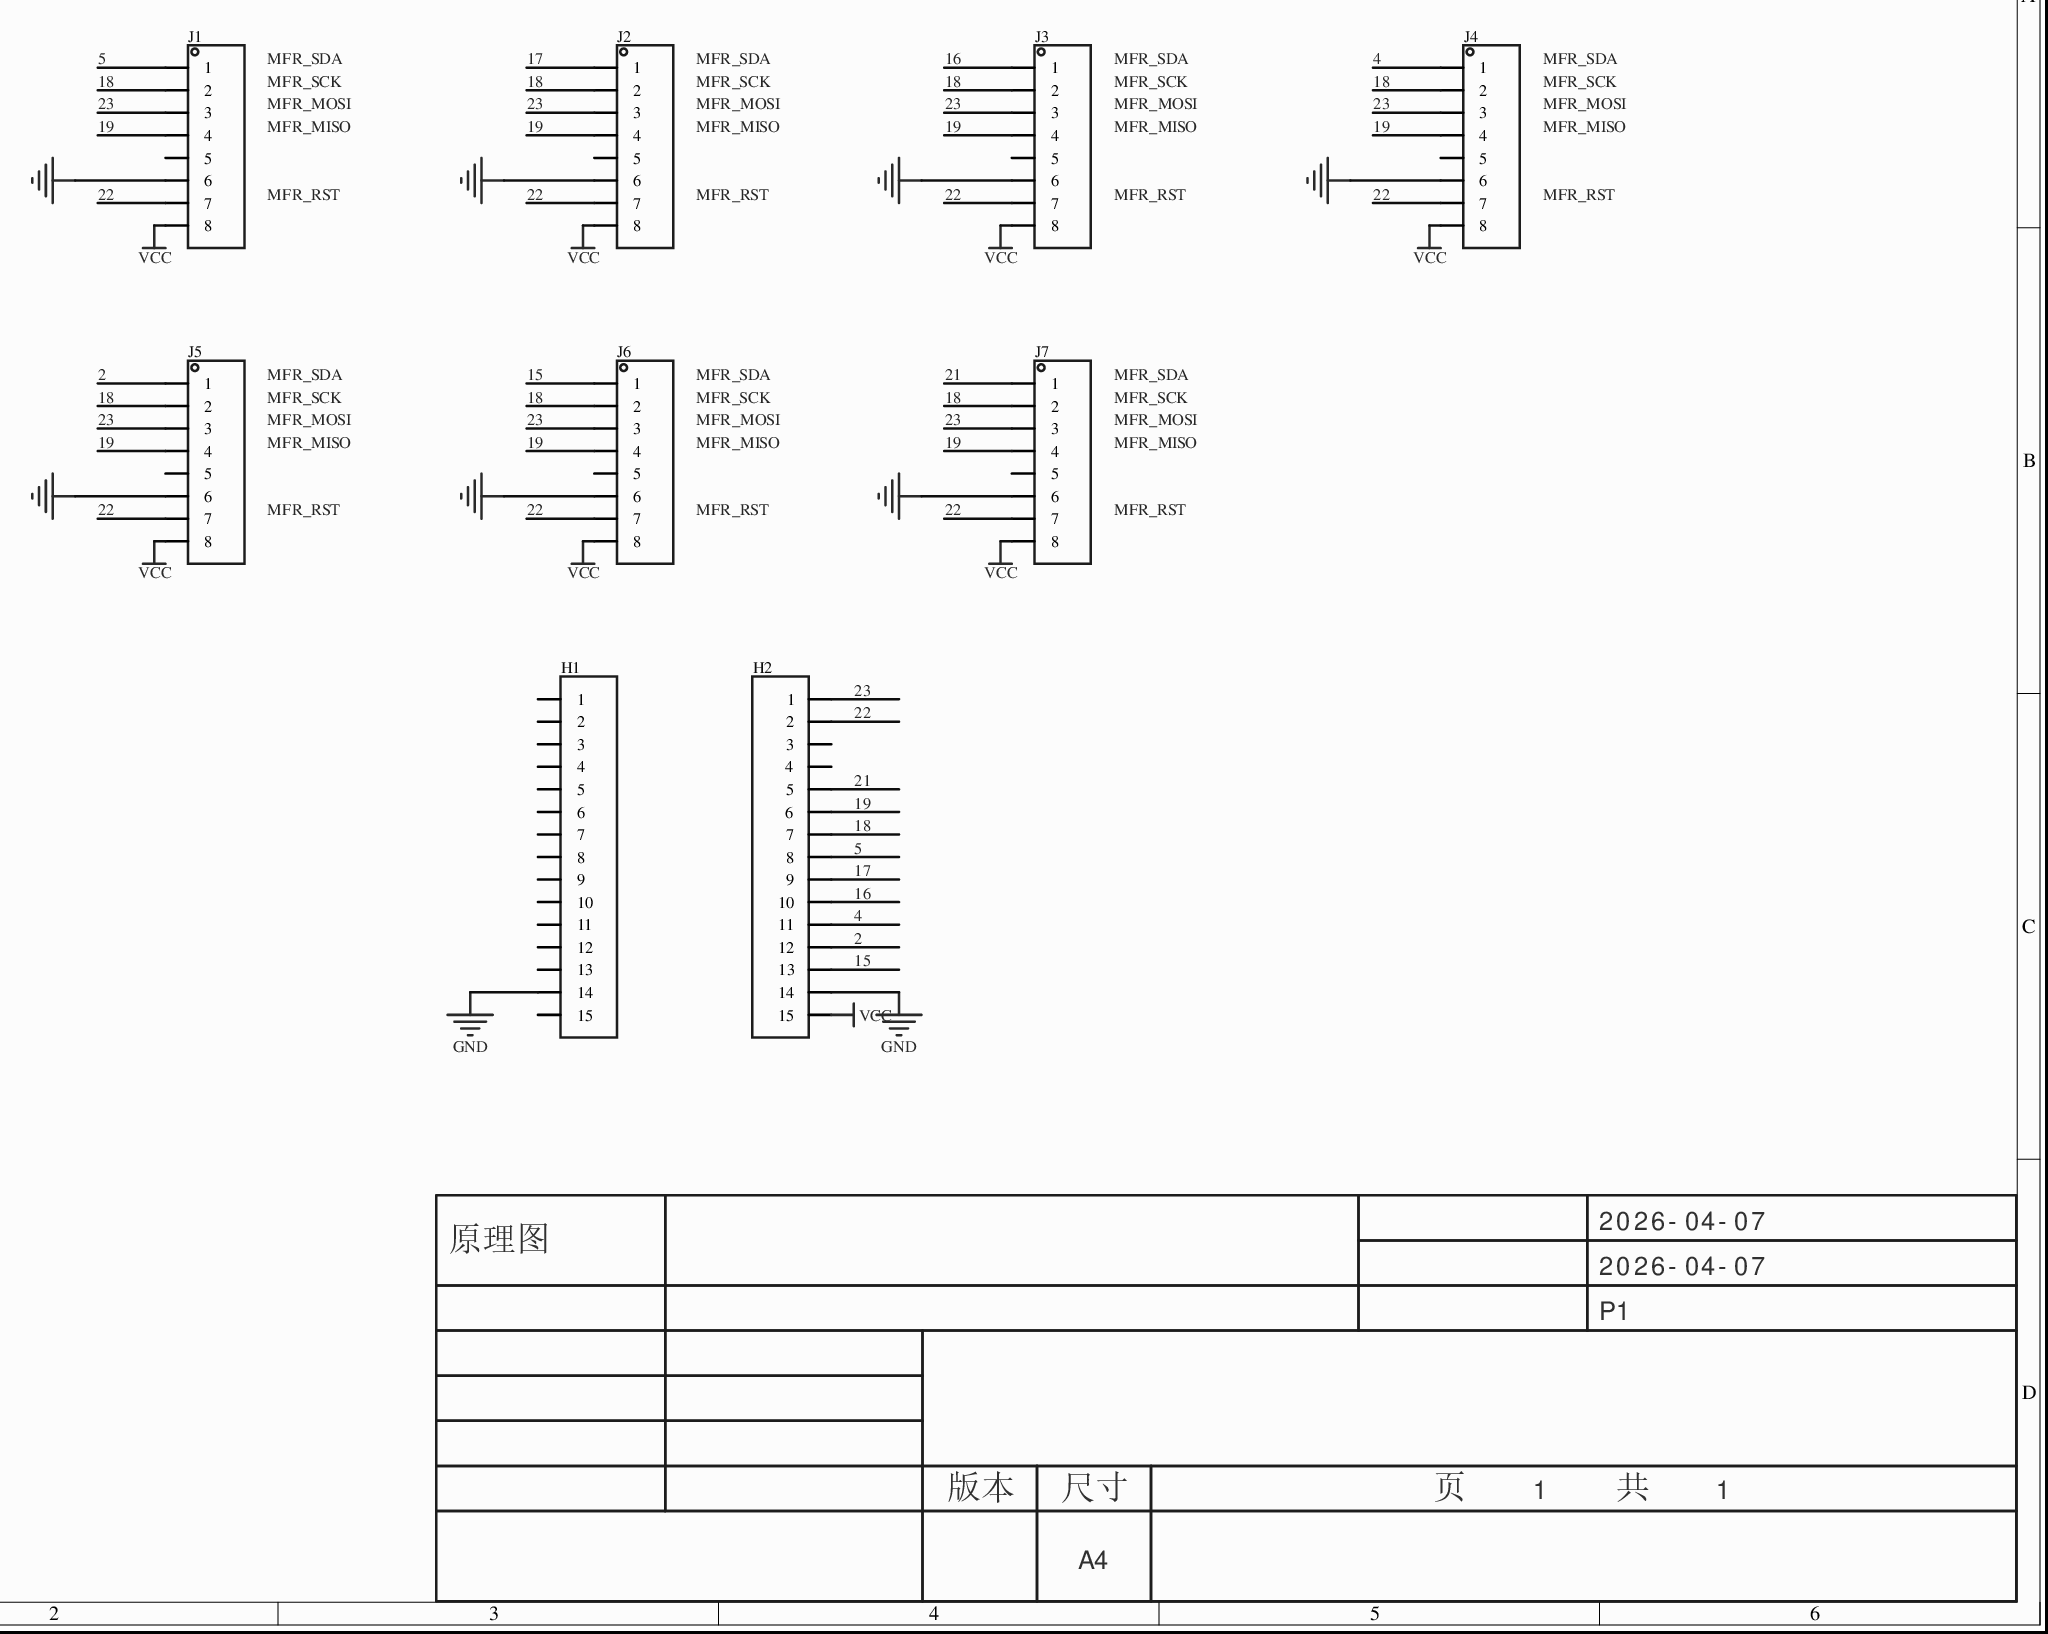
[diagram p0: MISC49852-3.schdoc]
# Altium project MISC49852-2.PrjPcb
1 sheet, 9 parts. Net scope: global (net labels, ports and power ports of the same name join across sheets).
Board file: MISC49852.pcbdoc

## Sheet MISC49852-3.schdoc
size 297 x 209 mm; Version: V1.0; @Project Name: MISC49852; @Update Date: 2026-04-07; @Create Date: 2026-04-07; @Board Name: MISC49852; @Create Time: 16:58:09; @Page Count: 1; @Page No: 1; @Schematic Name: MISC49852; @Update Time: 16:58:09; Size: A4

### Parts
H1  (no value)  [HDR-TH_15P-P2.54-V-F-1]
H2  (no value)  [HDR-TH_15P-P2.54-V-F-1]
J1  (no value)  [HDR-TH_8P-P2.54-V-M]
J2  (no value)  [HDR-TH_8P-P2.54-V-M]
J3  (no value)  [HDR-TH_8P-P2.54-V-M]
J4  (no value)  [HDR-TH_8P-P2.54-V-M]
J5  (no value)  [HDR-TH_8P-P2.54-V-M]
J6  (no value)  [HDR-TH_8P-P2.54-V-M]
J7  (no value)  [HDR-TH_8P-P2.54-V-M]

### Nets
GND: H1.14 H2.14 J1.6 J2.6 J3.6 J4.6 J5.6 J6.6 J7.6
VCC: H2.15 J1.8 J2.8 J3.8 J4.8 J5.8 J6.8 J7.8
2: H2.12 J5.1
4: H2.11 J4.1
5: H2.8 J1.1
15: H2.13 J6.1
16: H2.10 J3.1
17: H2.9 J2.1
18: H2.7 J1.2 J2.2 J3.2 J4.2 J5.2 J6.2 J7.2
19: H2.6 J1.4 J2.4 J3.4 J4.4 J5.4 J6.4 J7.4
21: H2.5 J7.1
22: H2.2 J1.7 J2.7 J3.7 J4.7 J5.7 J6.7 J7.7
23: H2.1 J1.3 J2.3 J3.3 J4.3 J5.3 J6.3 J7.3

Not connected (* = marked no-connect by the designer): H1 1 2 3 4 5 6 7 8 9 10 11 12 13 15; H2 3 4; J1 5; J2 5; J3 5; J4 5; J5 5; J6 5; J7 5

### Notes on the sheet
- Labels drawn without touching a wire or pin: MFR_MISO, MFR_MOSI, MFR_RST, MFR_SCK, MFR_SDA
- 2026-04-07
- 原理图
- P1
- 版本
- 尺寸
- A4
- 页    1    共    1

### Library data of the parts
H1 H2 = HDR-F_2.54_1x15P: ConvertToPcb: yes; ModelId: 88d88d3d05774da49ce8fa2ce222e7100819f05c4eef4c71ace90d822a990e87; ModelTransform: 1515.745,94.488,0,0,0,0,0,0,-125.984; Symbol: HDR-F_2.54_1x15P; Device: HDR-F_2.54_1x15P; AddInBom: yes; SupplierPart: C124408; Supplier Footprint: 插件,; FootprintName: HDR-TH_15P-P2.54-V-F-1; ModelName: HDR-TH_15P-P2.54-V-F-1
J1-J7 = HDR-M_2.54_1x8P: Symbol: Header-Male-2.54_1x8; 3D Model: f5b96e27511e49e38545e53df2320202; 3D Model Transform: 807.87244,98.425,0,0,0,0,0,0,-118.11; ConvertToPcb: yes; Device: HDR-M_2.54_1x8P; Supplier Part: C124381; Supplier Footprint: 插件; AddInBom: yes; FootprintName: HDR-TH_8P-P2.54-V-M; ModelName: HDR-TH_8P-P2.54-V-M